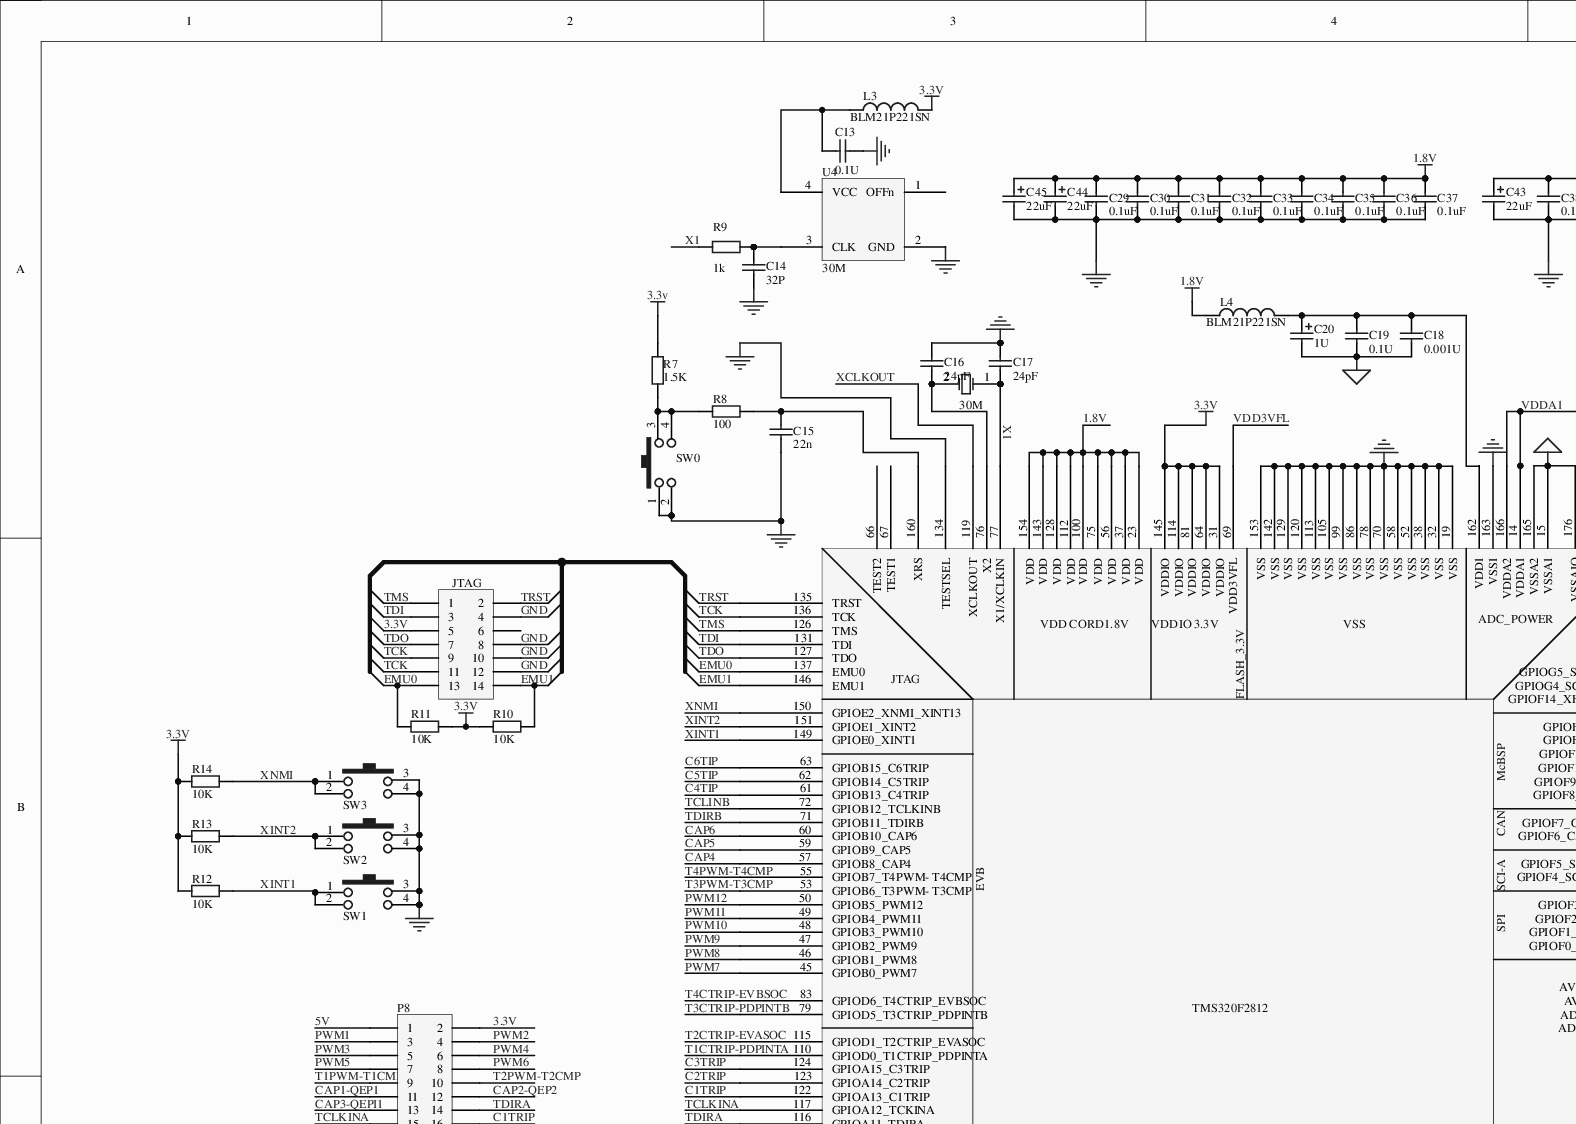
[diagram p0: MISC76198.SCHDOC, top left]
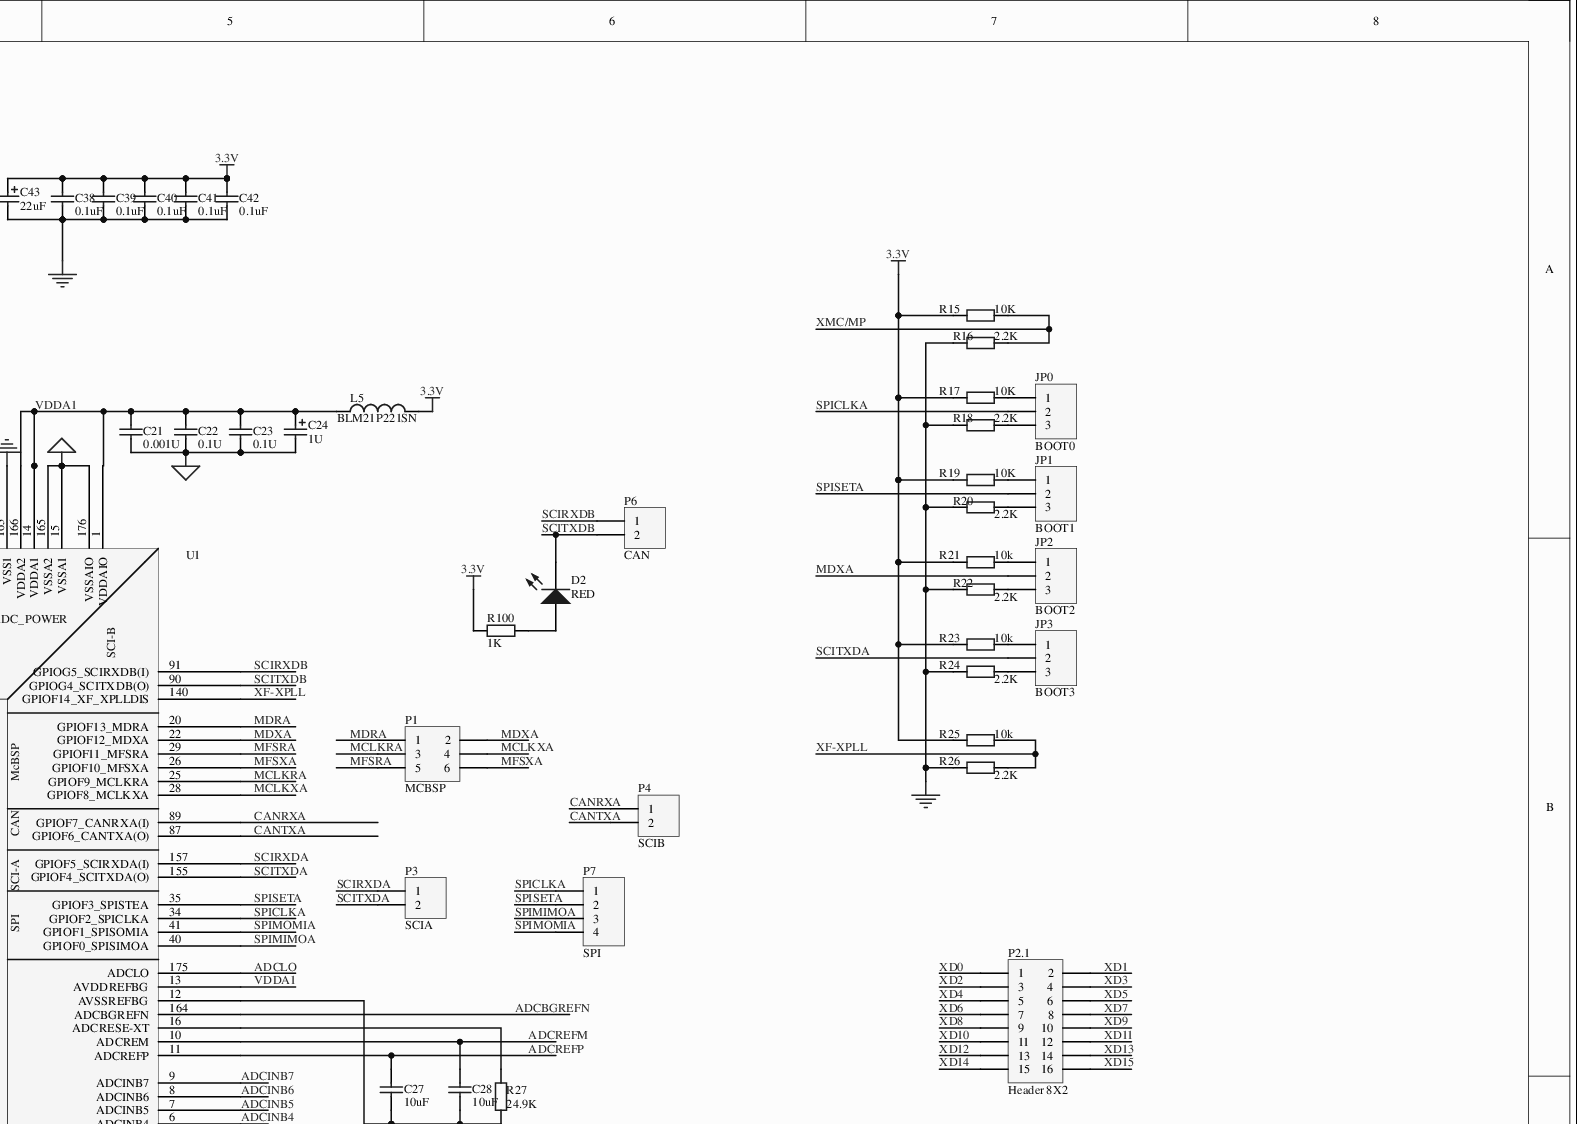
[diagram p1: MISC76198.SCHDOC, top right]
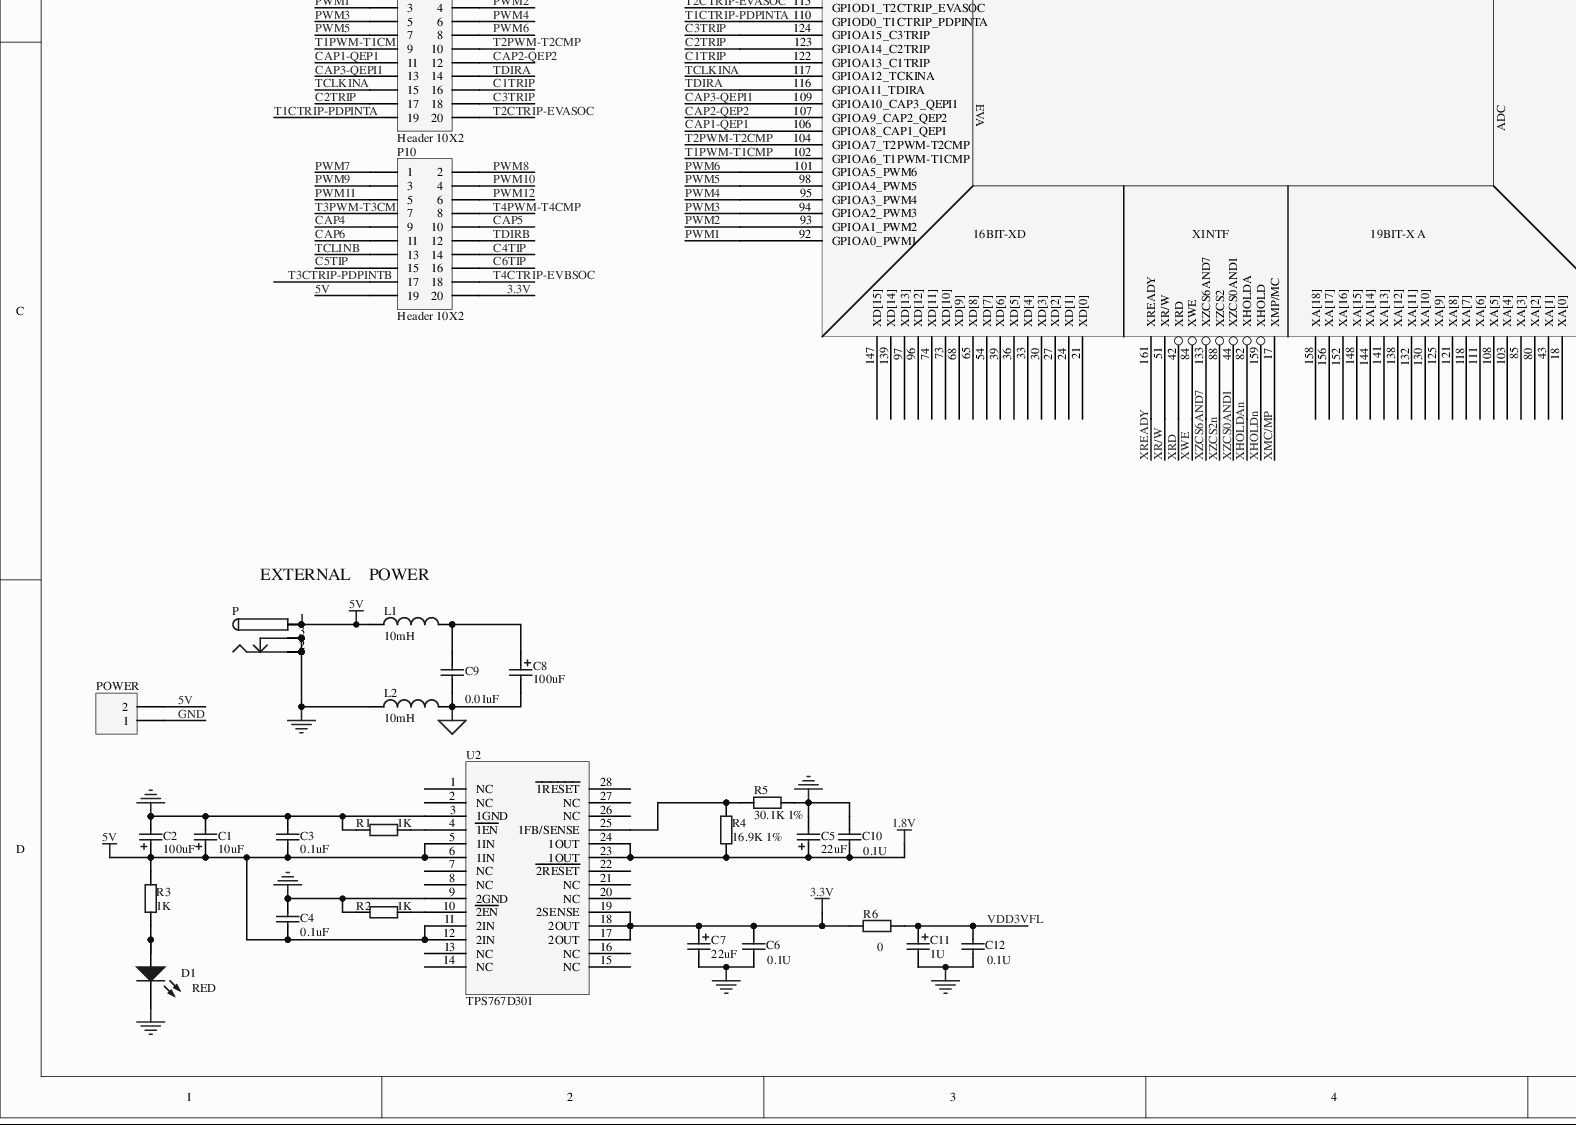
[diagram p2: MISC76198.SCHDOC, bottom left]
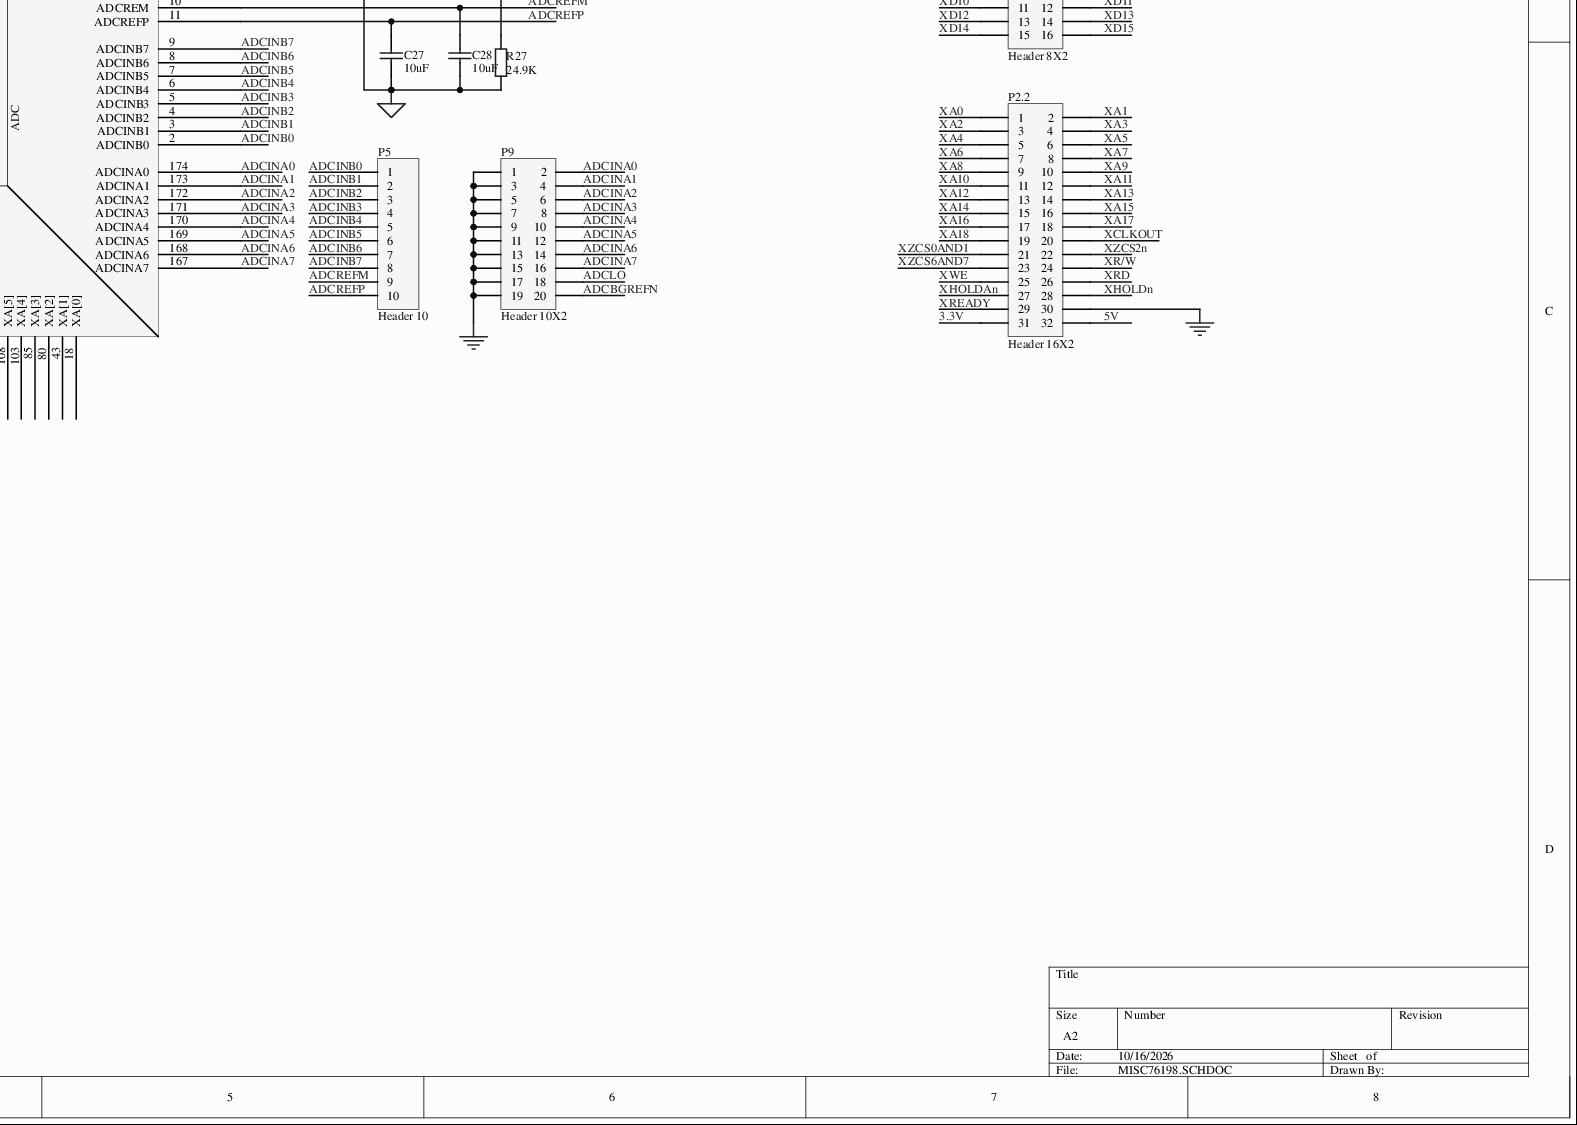
[diagram p3: MISC76198.SCHDOC, bottom right]
# Altium project MISC76198-3.PRJPCB
1 sheet, 104 parts. Net scope: global (net labels, ports and power ports of the same name join across sheets).
Board file: MISC76198.PCBDOC

## Sheet MISC76198.SCHDOC
size A2

### Parts
30M  XTAL  [TXAL]  (value not drawn)
C1  value 10uF  [C2]  (hidden comment: Cap Pol1)
C2  value 100uF  [C1]  (hidden comment: Cap Pol1)
C3  value 0.1uF  [0603]  (hidden comment: Cap)
C4  value 0.1uF  [0603]  (hidden comment: Cap)
C5  value 22uF  [C2]  (hidden comment: Cap Pol1)
C6  value 0.1U  [0603]  (hidden comment: Cap)
C7  value 22uF  [c2]  (hidden comment: Cap Pol1)
C8  value 100uF  [C1]  (hidden comment: Cap Pol1)
C9  value 0.01uF  [0603]  (hidden comment: Cap)
C10  value 0.1U  [0603]  (hidden comment: Cap)
C11  value 1U  [1210]  (hidden comment: Cap Pol1)
C12  value 0.1U  [0603]  (hidden comment: Cap)
C13  value 0.1U  [0603]  (hidden comment: Cap)
C14  value 32P  [0603]  (hidden comment: Cap)
C15  value 22n  [0603]  (hidden comment: Cap)
C16  value 24pF  [0603]  (hidden comment: Cap Semi)
C17  value 24pF  [0603]  (hidden comment: Cap Semi)
C18  value 0.001U  [0603]  (hidden comment: Cap Semi)
C19  value 0.1U  [0603]  (hidden comment: Cap Semi)
C20  value 1U  [0805]  (hidden comment: Cap Pol1)
C21  value 0.001U  [0603]  (hidden comment: Cap Semi)
C22  value 0.1U  [0603]  (hidden comment: Cap Semi)
C23  value 0.1U  [0603]  (hidden comment: Cap Semi)
C24  value 1U  [0805]  (hidden comment: Cap Pol1)
C27  value 10uF  [0603]  (hidden comment: Cap)
C28  value 10uF  [0603]  (hidden comment: Cap)
C29  0.1uF  [0603]
C30  0.1uF  [0603]
C31  0.1uF  [0603]
C32  0.1uF  [0603]
C33  0.1uF  [0603]
C34  0.1uF  [0603]
C35  0.1uF  [0603]
C36  0.1uF  [0603]
C37  0.1uF  [0603]
C38  0.1uF  [0603]
C39  0.1uF  [0603]
C40  0.1uF  [0603]
C41  0.1uF  [0603]
C42  0.1uF  [0603]
C43  value 22uF  [1206]  (hidden comment: Cap Pol1)
C44  value 22uF  [1206]  (hidden comment: Cap Pol1)
C45  value 22uF  [1206]  (hidden comment: Cap Pol1)
D1  RED  [0603]
D2  RED  [0603]
JP0  BOOT0  [HDR1X3]
JP1  BOOT1  [HDR1X3]
JP2  BOOT2  [HDR1X3]
JP3  BOOT3  [HDR1X3]
JTAG  Header 7X2  [HDR2X7]  (value not drawn)
L1  value 10mH  [0805]  (hidden comment: Inductor)
L2  value 10mH  [0805]  (hidden comment: Inductor)
L3  value BLM21P221SN  [0805]  (hidden comment: Inductor)
L4  value BLM21P221SN  [0805]  (hidden comment: Inductor)
L5  value BLM21P221SN  [0805]  (hidden comment: Inductor)
P  PWR2.5  [KLD-0202]  (value not drawn)
P1  MCBSP  [HDR2X3]
P2.1  Header 8X2  [HDR2X8]
P2.2  Header 16X2  [HDR2X16]
P3  SCIA  [HDR1X2]
P4  SCIB  [HDR1X2]
P5  Header 10  [HDR1X10]
P6  CAN  [HDR1X2]
P7  SPI  [HDR1X4]
P8  Header 10X2  [HDR2X10]
P9  Header 10X2  [HDR2X10]
P10  Header 10X2  [HDR2X10]
POWER  Header 2  [HDR1X2]  (value not drawn)
R1  value 1K  [0603]  (hidden comment: Res2)
R2  value 1K  [0603]  (hidden comment: Res2)
R3  value 1K  [0603]  (hidden comment: Res2)
R4  value 16.9K 1%  [0603]  (hidden comment: Res2)
R5  value 30.1K 1%  [0603]  (hidden comment: Res2)
R6  value 0  [0603]  (hidden comment: Res2)
R7  1.5K  [0603]
R8  100  [0603]
R9  1k  [0603]
R10  value 10K  [0603]  (hidden comment: Res2)
R11  value 10K  [0603]  (hidden comment: Res2)
R12  value 10K  [0603]  (hidden comment: Res2)
R13  value 10K  [0603]  (hidden comment: Res2)
R14  value 10K  [0603]  (hidden comment: Res2)
R15  10K  [0603]
R16  value 2.2K  [0603]  (hidden comment: 1k)
R17  10K  [0603]
R18  2.2K  [0603]
R19  10K  [0603]
R20  2.2K  [0603]
R21  10k  [0603]
R22  2.2K  [0603]
R23  10k  [0603]
R24  2.2K  [0603]
R25  10k  [0603]
R26  2.2K  [0603]
R27  24.9K  [0603]
R100  value 1K  [0603]  (hidden comment: Res2)
SW0  KEY4  [key]  (value not drawn)
SW1  KEY4  [key]  (value not drawn)
SW2  KEY4  [key]  (value not drawn)
SW3  KEY4  [key]  (value not drawn)
U1  TMS320F2812  [QFP176]  (value not drawn)
U2  TPS767D301  [TSOP28(0.65mm)]
U4  30M  [CRYSTAL1]

### Nets
1.8V: C5.1 C10.1 C29.1 C30.2 C31.2 C32.2 C33.2 C34.2 C35.2 C36.2 C37.2 C44.1 C45.1 L4.1 R4.1 U1.23(VDD) U1.37(VDD) U1.56(VDD) U1.75(VDD) U1.100(VDD) U1.112(VDD) U1.128(VDD) U1.143(VDD) U1.154(VDD) U2.23(1OUT) U2.24(1OUT)
3.3V: C6.2 C7.1 C38.2 C39.2 C40.2 C41.1 C42.2 C43.1 JTAG.5 L3.2 L5.2 P2.2.31 P8.2 P10.20 R6.2 R7.2 R10.2 R11.2 R12.1 R13.1 R14.1 R15.1 R17.1 R19.1 R21.1 R23.1 R25.1 R100.1 U1.31(VDDIO) U1.64(VDDIO) U1.81(VDDIO) U1.114(VDDIO) U1.145(VDDIO) U2.17(2OUT) U2.18(2OUT) U2.19(2SENSE)
5V: C1.1 C2.1 C3.1 C4.2 L1.1 P.1 P.1A P.1B P2.2.32 P8.1 P10.19 POWER.2 R3.2 U2.5(1IN) U2.6(1IN) U2.11(2IN) U2.12(2IN)
AGND: C8.2 C9.1 C18.1 C19.1 C20.2 C21.1 C22.1 C23.1 C24.2 C27.2 C28.2 L2.2 R27.2 U1.12(AVSSREFBG) U1.15(VSSA1) U1.165(VSSA2) U1.176(VSSAIO)
GND: C1.2 C2.2 C3.2 C4.1 C5.2 C6.1 C7.2 C10.2 C11.2 C12.1 C13.1 C14.1 C15.1 C16.1 C17.2 C29.2 C30.1 C31.1 C32.1 C33.1 C34.1 C35.1 C36.1 C37.1 C38.1 C39.1 C40.1 C41.2 C42.1 C43.2 C44.2 C45.2 D1.2(K) JTAG.4 JTAG.8 JTAG.10 JTAG.12 L2.1 P.2 P.2A P.2B P.3 P.3A P.3B P2.2.30 P9.1 P9.3 P9.5 P9.7 P9.9 P9.11 P9.13 P9.15 P9.17 P9.19 POWER.1 R1.1 R2.1 R5.2 R16.1 R18.1 R20.1 R22.1 R24.1 R26.1 SW0.1 SW0.2 SW1.3 SW1.4 SW2.3 SW2.4 SW3.3 SW3.4 U1.19(VSS) U1.32(VSS) U1.38(VSS) U1.52(VSS) U1.58(VSS) U1.70(VSS) U1.78(VSS) U1.86(VSS) U1.99(VSS) U1.105(VSS) U1.113(VSS) U1.120(VSS) U1.129(VSS) U1.134(TESTSEL) U1.142(VSS) U1.153(VSS) U1.163(VSS1) U2.3(1GND) U2.9(2GND) U4.2(GND)
ADCBGREFN: P9.20 U1.164(ADCBGREFN)
ADCINA0: P9.2 U1.174(ADCINA0)
ADCINA1: P9.4 U1.173(ADCINA1)
ADCINA2: P9.6 U1.172(ADCINA2)
ADCINA3: P9.8 U1.171(ADCINA3)
ADCINA4: P9.10 U1.170(ADCINA4)
ADCINA5: P9.12 U1.169(ADCINA5)
ADCINA6: P9.14 U1.168(ADCINA6)
ADCINA7: P9.16 U1.167(ADCINA7)
ADCINB0: P5.1 U1.2(ADCINB0)
ADCINB1: P5.2 U1.3(ADCINB1)
ADCINB2: P5.3 U1.4(ADCINB2)
ADCINB3: P5.4 U1.5(ADCINB3)
ADCINB4: P5.5 U1.6(ADCINB4)
ADCINB5: P5.6 U1.7(ADCINB5)
ADCINB6: P5.7 U1.8(ADCINB6)
ADCINB7: P5.8 U1.9(ADCINB7)
ADCLO: P9.18 U1.175(ADCLO)
ADCREFM: C28.1 P5.9 U1.10(ADCREM)
ADCREFP: C27.1 P5.10 U1.11(ADCREFP)
C1TRIP: P8.16 U1.122(GPIOA13_C1TRIP)
C2TRIP: P8.17 U1.123(GPIOA14_C2TRIP)
C3TRIP: P8.18 U1.124(GPIOA15_C3TRIP)
C4TIP: P10.14 U1.61(GPIOB13_C4TRIP)
C5TIP: P10.15 U1.62(GPIOB14_C5TRIP)
C6TIP: P10.16 U1.63(GPIOB15_C6TRIP)
CANRXA: P4.1 U1.89(GPIOF7_CANRXA(I))
CANTXA: P4.2 U1.87(GPIOF6_CANTXA(O))
CAP1-QEP1: P8.11 U1.106(GPIOA8_CAP1_QEP1)
CAP2-QEP2: P8.12 U1.107(GPIOA9_CAP2_QEP2)
CAP3-QEPI1: P8.13 U1.109(GPIOA10_CAP3_QEPI1)
CAP4: P10.9 U1.57(GPIOB8_CAP4)
CAP5: P10.10 U1.59(GPIOB9_CAP5)
CAP6: P10.11 U1.60(GPIOB10_CAP6)
EMU0: JTAG.13 R11.1 U1.137(EMU0)
EMU1: JTAG.14 R10.1 U1.146(EMU1)
MCLKRA: P1.3 U1.25(GPIOF9_MCLKRA)
MCLKXA: P1.4 U1.28(GPIOF8_MCLKXA)
MDRA: P1.1 U1.20(GPIOF13_MDRA)
MDXA: JP2.2 P1.2 U1.22(GPIOF12_MDXA)
MFSRA: P1.5 U1.29(GPIOF11_MFSRA)
MFSXA: P1.6 U1.26(GPIOF10_MFSXA)
PWM1: P8.3 U1.92(GPIOA0_PWM1)
PWM2: P8.4 U1.93(GPIOA1_PWM2)
PWM3: P8.5 U1.94(GPIOA2_PWM3)
PWM4: P8.6 U1.95(GPIOA3_PWM4)
PWM5: P8.7 U1.98(GPIOA4_PWM5)
PWM6: P8.8 U1.101(GPIOA5_PWM6)
PWM7: P10.1 U1.45(GPIOB0_PWM7)
PWM8: P10.2 U1.46(GPIOB1_PWM8)
PWM9: P10.3 U1.47(GPIOB2_PWM9)
PWM10: P10.4 U1.48(GPIOB3_PWM10)
PWM11: P10.5 U1.49(GPIOB4_PWM11)
PWM12: P10.6 U1.50(GPIOB5_PWM12)
SCIRXDA: P3.1 U1.157(GPIOF5_SCIRXDA(I))
SCIRXDB: P6.1 U1.91(GPIOG5_SCIRXDB(I))
SCITXDA: JP3.2 P3.2 U1.155(GPIOF4_SCITXDA(O))
SCITXDB: D2.2(K) P6.2 U1.90(GPIOG4_SCITXDB(O))
SPICLKA: JP0.2 P7.1 U1.34(GPIOF2_SPICLKA)
SPIMIMOA: P7.3 U1.40(GPIOF0_SPISIMOA)
SPIMOMIA: P7.4 U1.41(GPIOF1_SPISOMIA)
SPISETA: JP1.2 P7.2 U1.35(GPIOF3_SPISTEA)
T1CTRIP-PDPINTA: P8.19 U1.110(GPIOD0_T1CTRIP_PDPINTA)
T1PWM-T1CMP: P8.9 U1.102(GPIOA6_T1PWM-T1CMP)
T2CTRIP-EVASOC: P8.20 U1.115(GPIOD1_T2CTRIP_EVASOC)
T2PWM-T2CMP: P8.10 U1.104(GPIOA7_T2PWM-T2CMP)
T3CTRIP-PDPINTB: P10.17 U1.79(GPIOD5_T3CTRIP_PDPINTB)
T3PWM-T3CMP: P10.7 U1.53(GPIOB6_T3PWM-_T3CMP)
T4CTRIP-EVBSOC: P10.18 U1.83(GPIOD6_T4CTRIP_EVBSOC)
T4PWM-T4CMP: P10.8 U1.55(GPIOB7_T4PWM-_T4CMP)
TCK: JTAG.9 JTAG.11 U1.136(TCK)
TCLINB: P10.13 U1.72(GPIOB12_TCLKINB)
TCLKINA: P8.15 U1.117(GPIOA12_TCKINA)
TDI: JTAG.3 U1.131(TDI)
TDIRA: P8.14 U1.116(GPIOA11_TDIRA)
TDIRB: P10.12 U1.71(GPIOB11_TDIRB)
TDO: JTAG.7 U1.127(TDO)
TMS: JTAG.1 U1.126(TMS)
TRST: JTAG.2 U1.135(TRST)
VDD3VFL: C11.1 C12.2 R6.1 U1.69(VDD3VFL)
VDDA1: C21.2 C22.2 C23.2 C24.1 L5.1 U1.1(VDDAIO) U1.13(AVDDREFBG) U1.14(VDDA1) U1.166(VDDA2)
X1: 30M.1(OSC1) C17.1 R9.1 U1.77(X1/XCLKIN)
XA0: P2.2.1
XA1: P2.2.2
XA2: P2.2.3
XA3: P2.2.4
XA4: P2.2.5
XA5: P2.2.6
XA6: P2.2.7
XA7: P2.2.8
XA8: P2.2.9
XA9: P2.2.10
XA10: P2.2.11
XA11: P2.2.12
XA12: P2.2.13
XA13: P2.2.14
XA14: P2.2.15
XA15: P2.2.16
XA16: P2.2.17
XA17: P2.2.18
XA18: P2.2.19
XCLKOUT: P2.2.20 U1.119(XCLKOUT)
XD0: P2.1.1
XD1: P2.1.2
XD2: P2.1.3
XD3: P2.1.4
XD4: P2.1.5
XD5: P2.1.6
XD6: P2.1.7
XD7: P2.1.8
XD8: P2.1.9
XD9: P2.1.10
XD10: P2.1.11
XD11: P2.1.12
XD12: P2.1.13
XD13: P2.1.14
XD14: P2.1.15
XD15: P2.1.16
XF-XPLL: R25.2 R26.2 U1.140(GPIOF14_XF_XPLLDIS)
XHOLDAn: P2.2.27 U1.82(XHOLDA)
XHOLDn: P2.2.28 U1.159(XHOLD)
XINT1: R12.2 SW1.1 SW1.2 U1.149(GPIOE0_XINT1)
XINT2: R13.2 SW2.1 SW2.2 U1.151(GPIOE1_XINT2)
XMC/MP: R15.2 R16.2 U1.17(XMP/MC)
XNMI: R14.2 SW3.1 SW3.2 U1.150(GPIOE2_XNMI_XINT13)
XR/W: P2.2.24 U1.51(XR/W)
XRD: P2.2.26 U1.42(XRD)
XREADY: P2.2.29 U1.161(XREADY)
XWE: P2.2.25 U1.84(XWE)
XZCS0AND1: P2.2.21 U1.44(XZCS0AND1)
XZCS2n: P2.2.22 U1.88(XZCS2)
XZCS6AND7: P2.2.23 U1.133(XZCS6AND7)
Net30M_2: 30M.2(OSC2) C16.2 U1.76(X2)
NetC8_1: C8.1 C9.2 L1.2
NetC13_2: C13.2 L3.1 U4.4(VCC)
NetC14_2: C14.2 R9.2 U4.3(CLK)
NetC15_2: C15.2 R8.2 U1.160(XRS)
NetC18_2: C18.2 C19.2 C20.1 L4.2 U1.162(VDD1)
NetD1_1: D1.1(A) R3.1
NetD2_1: D2.1(A) R100.2
NetJP0_1: JP0.1 R17.2
NetJP0_3: JP0.3 R18.2
NetJP1_1: JP1.1 R19.2
NetJP1_3: JP1.3 R20.2
NetJP2_1: JP2.1 R21.2
NetJP2_3: JP2.3 R22.2
NetJP3_1: JP3.1 R23.2
NetJP3_3: JP3.3 R24.2
NetR1_2: R1.2 U2.4(~{1EN})
NetR2_2: R2.2 U2.10(~{2EN})
NetR4_2: R4.2 R5.1 U2.25(1FB/SENSE)
NetR7_1: R7.1 R8.1 SW0.3 SW0.4
NetR27_1: R27.1 U1.16(ADCRESE-XT)

Not connected (* = marked no-connect by the designer): JTAG 6*; U1 18(XA[0]) 21(XD[0]) 24(XD[1]) 27(XD[2]) 30(XD[3]) 33(XD[4]) 36(XD[5]) 39(XD[6]) 43(XA[1]) 54(XD[7]) 65(XD[8]) 66(TEST2) 67(TEST1) 68(XD[9]) 73(XD[10]) 74(XD[11]) 80(XA[2]) 85(XA[3]) 96(XD[12]) 97(XD[13]) 103(XA[4]) 108(XA[5]) 111(XA[6]) 118(XA[7]) 121(XA[8]) 125(XA[9]) 130(XA[10]) 132(XA[11]) 138(XA[12]) 139(XD[14]) 141(XA[13]) 144(XA[14]) 147(XD[15]) 148(XA[15]) 152(XA[16]) 156(XA[17]) 158(XA[18]); U2 1(NC)* 2(NC)* 7(NC)* 8(NC)* 13(NC)* 14(NC)* 15(NC)* 16(NC)* 20(NC)* 21(NC)* 22(~{2RESET})* 26(NC)* 27(NC)* 28(~{1RESET})*; U4 1(OFFn)

### Notes on the sheet
- EXTERNAL    POWER

### Library data of the parts
30M = XTAL: Crystal Oscillator; Published: 8-Jun-2000; LatestRevisionDate: 17-Jul-2002; LatestRevisionNote: Re-released for DXP Platform.; Publisher: Altium Limited
C1 C2 C5 C7 C8 C11 C20 C24 C43-C45 = Cap Pol1: Polarized Capacitor (Radial); Published: 8-Jun-2000; Revision: July-2002: Re-released for DXP Platform.; Publisher: Altium Limited
C3 C4 C6 C9 C10 C12-C15 C27 C28 = Cap: Capacitor; Published: 8-Jun-2000; Publisher: Altium Limited
  C3 C4 C9 C27 C28: Revision: July-2002: Re-released for DXP Platform.
  C6 C10 C12-C15: LatestRevisionDate: 17-Jul-2002; LatestRevisionNote: Re-released for DXP Platform.
C16-C19 C21-C23 = Cap Semi: Capacitor (Semiconductor SIM Model); Published: 8-Jun-2000; LatestRevisionDate: 17-Jul-2002; LatestRevisionNote: Re-released for DXP Platform.; PackageReference: C1206; Publisher: Altium Limited
C29-C42 = Cap: Capacitor; Value: 100pF; Published: 8-Jun-2000; LatestRevisionDate: 17-Jul-2002; LatestRevisionNote: Re-released for DXP Platform.; Publisher: Altium Limited
D1 D2 = HLMA-PG00-N0011: Subminiature High Performance AlInGaP LED Lamp; Package Information: Latest Revision: 19-Apr-2001; Min. Intensity: 25mcd; PCB Layout: Complies with manufacturer's recommendation.; Published: 11-Dec-2002; Datasheet: Latest Revision: 24-Oct-2001; Package Reference: 2.2X2.1X2.2; Colour: Red; Publisher: Altium Limited
JP0-JP3 = Header 3: Header, 3-Pin; LatestRevisionDate: 17-Jul-2002; LatestRevisionNote: Re-released for DXP Platform.; Publisher: Altium Limited
JTAG = Header 7X2: Header, 7-Pin, Dual row; Revision: 17-Jul-2002: Re-released for DXP Platform.; Publisher: Altium Limited
P = PWR2.5: Low Voltage Power Supply Connector; Published: 17-Dec-2003; Datasheet: Latest Revision: 09-May-2002; Publisher: Altium Limited
P1 = Header 3X2: Header, 3-Pin, Dual row; LatestRevisionDate: 17-Jul-2002; LatestRevisionNote: Re-released for DXP Platform.; Publisher: Altium Limited
P2.1 = Header 8X2: Header, 8-Pin, Dual row; LatestRevisionDate: 17-Jul-2002; LatestRevisionNote: Re-released for DXP Platform.; Publisher: Altium Limited
P2.2 = Header 16X2: Header, 16-Pin, Dual row; LatestRevisionDate: 17-Jul-2002; LatestRevisionNote: Re-released for DXP Platform.; Publisher: Altium Limited
P3 P4 P6 POWER = Header 2: Header, 2-Pin; Publisher: Altium Limited
  P3 P4 P6: LatestRevisionDate: 17-Jul-2002; LatestRevisionNote: Re-released for DXP Platform.
  POWER: Revision: 17-Jul-2002: Re-released for DXP Platform.
P5 = Header 10: Header, 10-Pin; LatestRevisionDate: 17-Jul-2002; LatestRevisionNote: Re-released for DXP Platform.; Publisher: Altium Limited
P7 = Header 4: Header, 4-Pin; LatestRevisionDate: 17-Jul-2002; LatestRevisionNote: Re-released for DXP Platform.; Publisher: Altium Limited
P8-P10 = Header 10X2: Header, 10-Pin, Dual row; LatestRevisionDate: 17-Jul-2002; LatestRevisionNote: Re-released for DXP Platform.; Publisher: Altium Limited
R1-R6 R9-R16 R27 R100 = Res2: Resistor; Published: 8-Jun-2000; Publisher: Altium Limited
  R1-R6 R10-R14 R100: Revision: July-2002: Re-released for DXP Platform.
  R9: LatestRevisionDate: 17-Jul-2002; LatestRevisionNote: Re-released for DXP Platform.; Value: 1K
  R15: LatestRevisionDate: 17-Jul-2002; LatestRevisionNote: Re-released for DXP Platform.; Value: 10K
  R16: LatestRevisionDate: 17-Jul-2002; LatestRevisionNote: Re-released for DXP Platform.
  R27: LatestRevisionDate: 17-Jul-2002; LatestRevisionNote: Re-released for DXP Platform.; Value: 24.9K
R7 R8 R17-R26 = Res2: Resistor; Value: 1K; Published: 8-Jun-2000; LatestRevisionDate: 17-Jul-2002; LatestRevisionNote: Re-released for DXP Platform.; Publisher: Altium Limited
U2 = TPS73HD301
L1-L5 = Inductor: Published: 8-Jun-2000; Revision: July-2002: Re-released for DXP Platform.; Publisher: Altium Limited